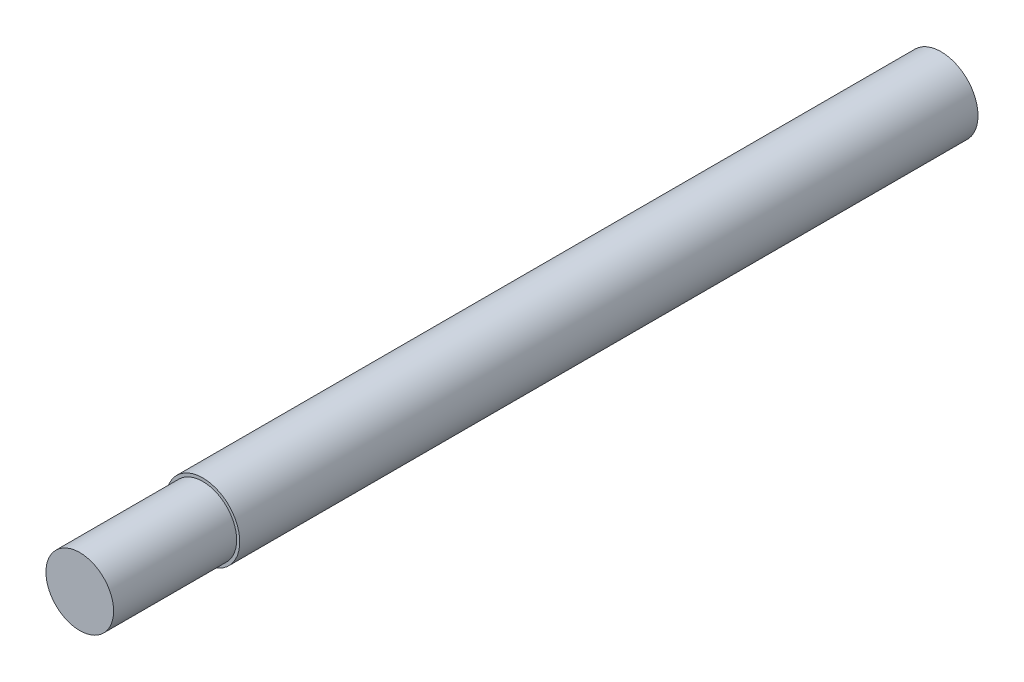
from build123d import *

# Parameters (mm, degrees)
SKETCH_1_R          = 6
EXTRUDE_3_DEPTH     = 70
SKETCH_3_R          = 6
SKETCH_3_R_2        = 5.5
CUT_EXTRUDE_1_DEPTH = 20


with BuildPart() as part:
    # 草图1 → 凸台-拉伸3 (new, symmetric)
    with BuildSketch(Plane.XY):
        Circle(SKETCH_1_R)
    extrude(amount=EXTRUDE_3_DEPTH, both=True)

    # 草图3 → 切除-拉伸1 (cut)
    with BuildSketch(Plane.XY.offset(70)):
        Circle(SKETCH_3_R)
        Circle(SKETCH_3_R_2, mode=Mode.SUBTRACT)
    extrude(amount=-CUT_EXTRUDE_1_DEPTH, mode=Mode.SUBTRACT)


solid = part.part
